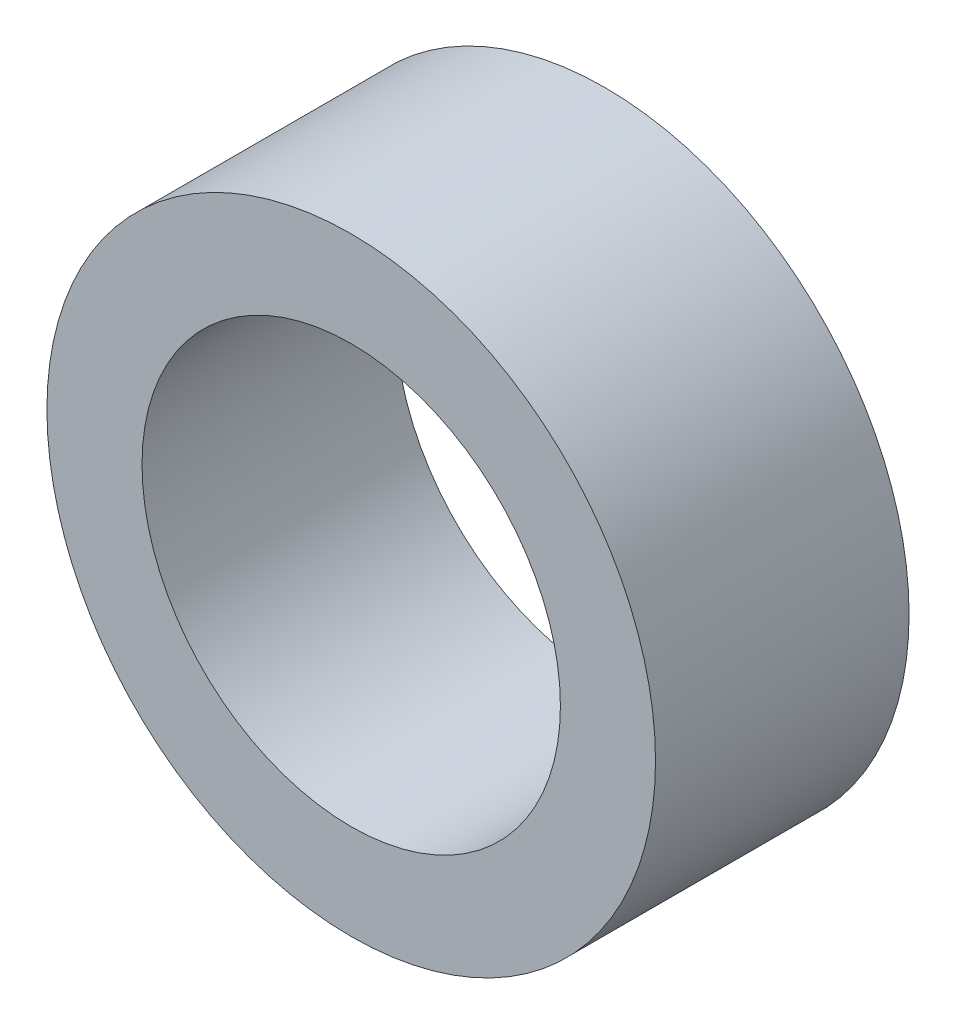
from build123d import *

# Parameters (mm, degrees)
SKETCH_1_R      = 12
SKETCH_1_R_2    = 8.25
EXTRUDE_1_DEPTH = 10


with BuildPart() as part:
    # 草图1 → 凸台-拉伸1 (new body)
    with BuildSketch(Plane.XY):
        Circle(SKETCH_1_R)
        Circle(SKETCH_1_R_2, mode=Mode.SUBTRACT)
    extrude(amount=EXTRUDE_1_DEPTH)


solid = part.part
